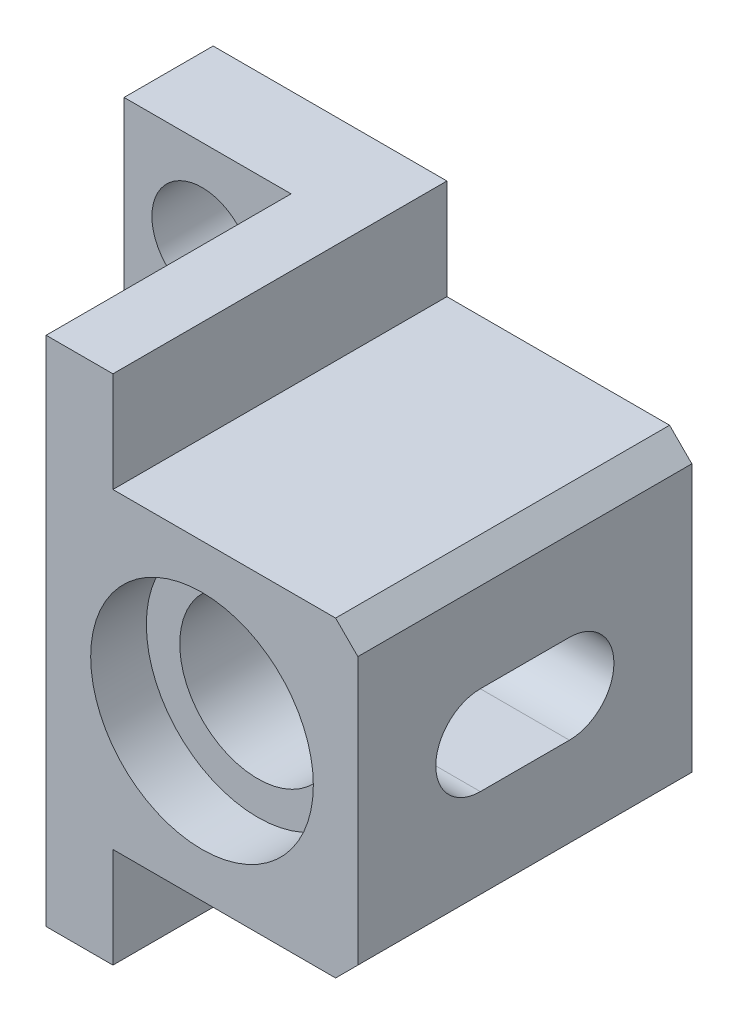
from build123d import *

# Parameters (mm, degrees)
SKETCH1_R           = 7
SKETCH1_R_2         = 4.5
BOSS_EXTRUDE1_DEPTH = 30
SKETCH2_W           = 15
SKETCH2_H           = 22
CUT_EXTRUDE1_DEPTH  = 59.976690311
CHAMFER1_SIZE       = 2
SKETCH3_R           = 10
CUT_EXTRUDE2_DEPTH  = 5
SKETCH4_W           = 5
SKETCH4_H           = 10
BOSS_EXTRUDE2_DEPTH = 4
CUT_EXTRUDE3_DEPTH  = 12


with BuildPart() as part:
    # Sketch1 → Boss-Extrude1 (new body)
    with BuildSketch(Plane.XY):
        Polygon((-21.5, 23), (-0.5, 23), (-0.5, 14), (21.5, 14), (21.5, -14), (-0.5, -14), (-0.5, -23), (-21.5, -23), align=None)
        with Locations((7.5, 0)):
            Circle(SKETCH1_R, mode=Mode.SUBTRACT)
        with Locations((-14.5, 15)):
            Circle(SKETCH1_R_2, mode=Mode.SUBTRACT)
        with Locations((-14.5, -15)):
            Circle(SKETCH1_R_2, mode=Mode.SUBTRACT)
    extrude(amount=BOSS_EXTRUDE1_DEPTH)

    # Sketch2 → Cut-Extrude1 (cut, through all)
    with BuildSketch(Plane(origin=(0, 23, 0), x_dir=(1, 0, 0), z_dir=(0, 1, 0))):
        with Locations((-14, -19)):
            Rectangle(SKETCH2_W, SKETCH2_H)
    extrude(amount=-CUT_EXTRUDE1_DEPTH, mode=Mode.SUBTRACT)

    # Chamfer1
    chamfer1_edges = [part.edges().sort_by_distance(p)[0] for p in [
        (21.5, 14, 15),
        (21.5, -14, 15),
    ]]
    chamfer(chamfer1_edges, length=CHAMFER1_SIZE)

    # Sketch3 → Cut-Extrude2 (cut)
    with BuildSketch(Plane.XY.offset(30)):
        with Locations((7.5, 0)):
            Circle(SKETCH3_R)
    extrude(amount=-CUT_EXTRUDE2_DEPTH, mode=Mode.SUBTRACT)

    # Sketch4 → Boss-Extrude2 (add)
    with BuildSketch(Plane.XY.offset(8)):
        with Locations((-19, 0)):
            Rectangle(SKETCH4_W, SKETCH4_H)
    extrude(amount=BOSS_EXTRUDE2_DEPTH)

    # Sketch5 → Cut-Extrude3 (cut)
    with BuildSketch(Plane(origin=(21.5, 0, 0), x_dir=(0, 0, -1), z_dir=(1, 0, 0))):
        with BuildLine():
            Line((-19, 4), (-11, 4))
            ThreePointArc((-11, 4), (-7, 0), (-11, -4))
            Line((-11, -4), (-19, -4))
            ThreePointArc((-19, -4), (-23, 0), (-19, 4))
        make_face()
    extrude(amount=-CUT_EXTRUDE3_DEPTH, mode=Mode.SUBTRACT)


solid = part.part
